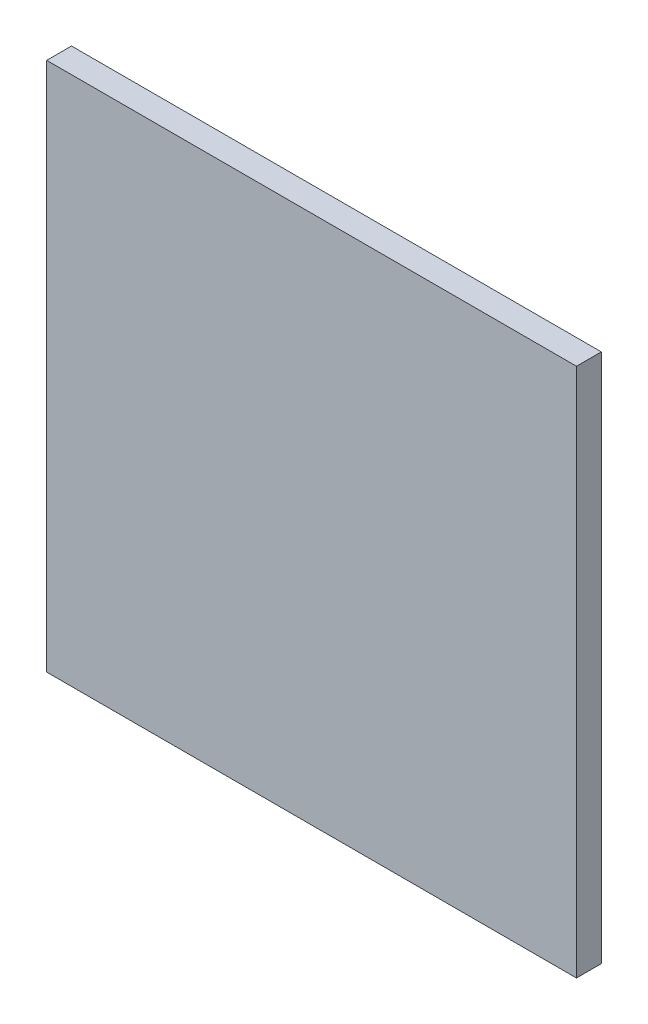
from build123d import *

# Parameters (mm, degrees)
SKETCH1_W           = 32
SKETCH1_H           = 32
BOSS_EXTRUDE1_DEPTH = 1.5


with BuildPart() as part:
    # Sketch1 → Boss-Extrude1 (new body)
    with BuildSketch(Plane.XY):
        Rectangle(SKETCH1_W, SKETCH1_H)
    extrude(amount=BOSS_EXTRUDE1_DEPTH)


solid = part.part
